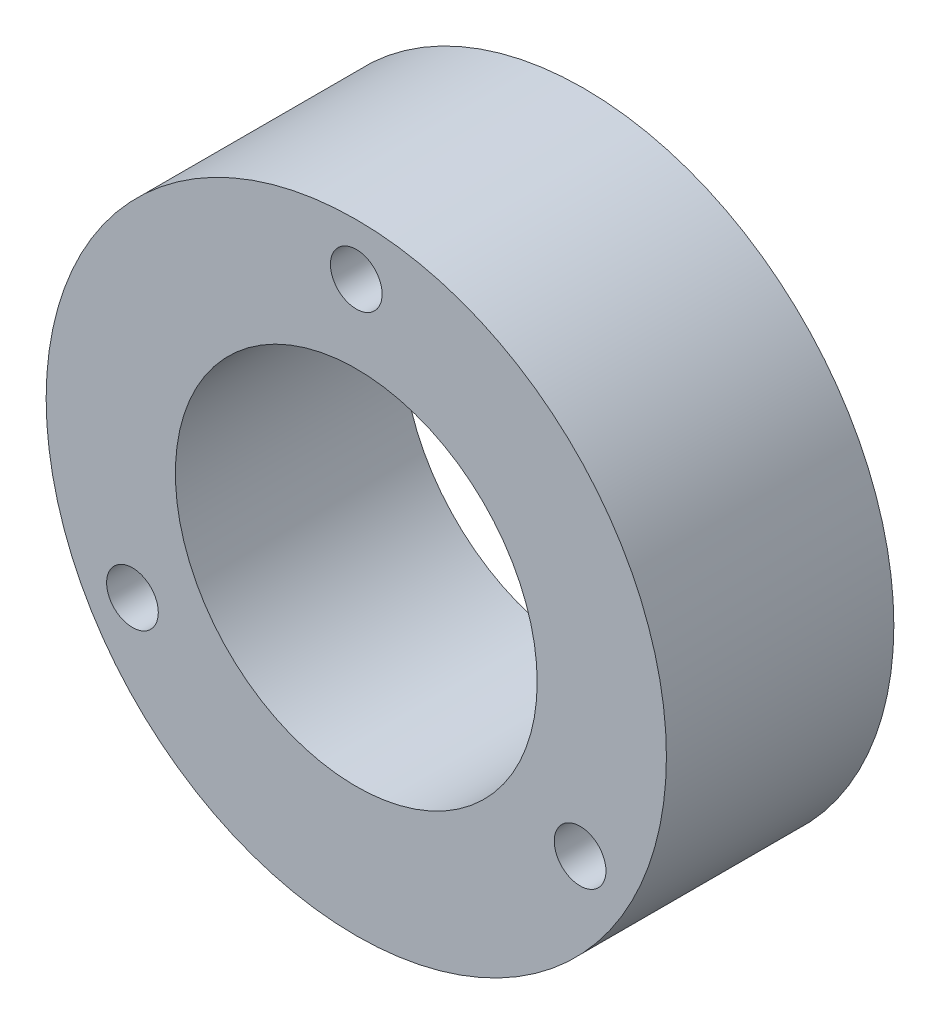
SolidWorks part; units mm, degrees
ref_plane "Front Plane" through (0, 0, 0) normal (0, 0, 1) x (1, 0, 0)
ref_plane "Top Plane" through (0, 0, 0) normal (0, 1, 0) x (1, 0, 0)
ref_plane "Right Plane" through (0, 0, 0) normal (1, 0, 0) x (0, 0, -1)
sketch "Sketch1" plane through (0, 0, 0) normal (0, 0, 1) x (1, 0, 0)
  circle A0 centre (0, 0) radius 17.5
  circle A1 centre (0, 0) radius 30
  circle A2 centre (0, 0) radius 25 construction
  circle A3 centre (0, 25) radius 2.5
  circle A4 centre (21.6506, -12.5) radius 2.5
  circle A5 centre (-21.6506, -12.5) radius 2.5
  point P14 (0, 0)
  dimension "D1" = 60
  dimension "D2" = 35
  dimension "D3" = 50
  dimension "D4" = 5
  dimension "D5" = 3
extrude "Boss-Extrude1" add sketch "Sketch1" along normal blind 22
